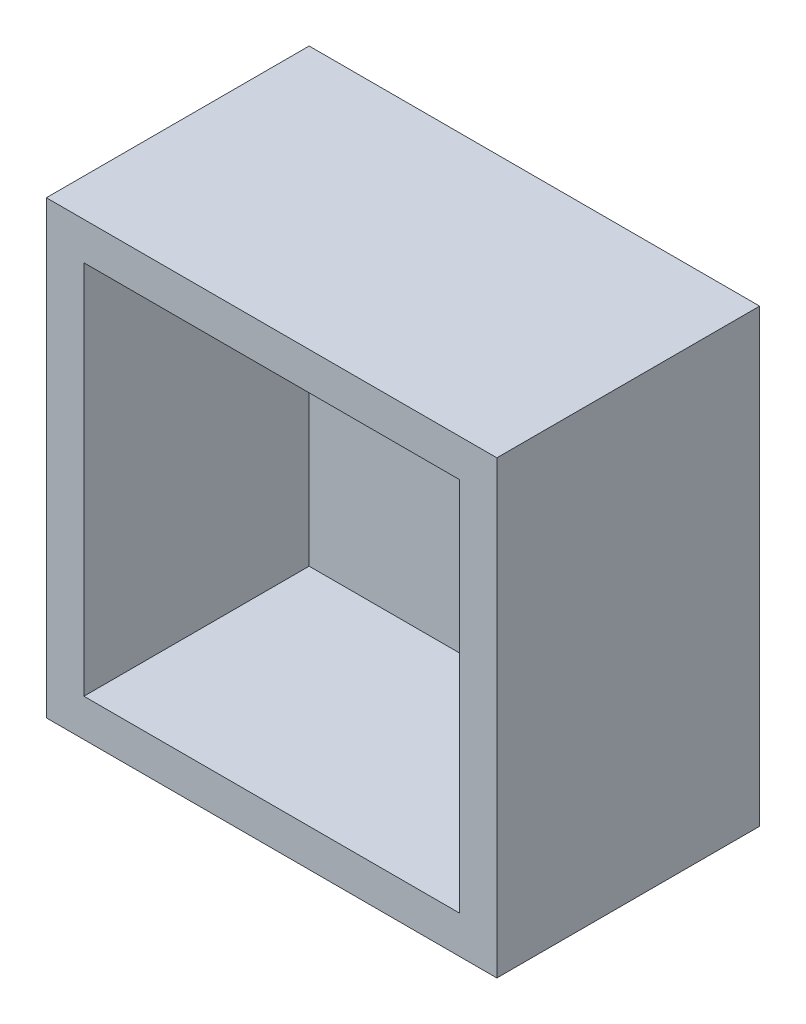
from build123d import *

# Parameters (mm, degrees)
SKETCH1_W           = 60
SKETCH1_H           = 60
BOSS_EXTRUDE1_DEPTH = 35
SHELL1_T            = -5


with BuildPart() as part:
    # Sketch1 → Boss-Extrude1 (new body)
    with BuildSketch(Plane.XY):
        with Locations((-88, 0)):
            Rectangle(SKETCH1_W, SKETCH1_H)
    extrude(amount=BOSS_EXTRUDE1_DEPTH)

    # Shell1
    shell1_openings = [part.faces().sort_by_distance(p)[0] for p in [
        (-88, 0, 35),
    ]]
    offset(amount=SHELL1_T, openings=shell1_openings, kind=Kind.INTERSECTION)


solid = part.part
